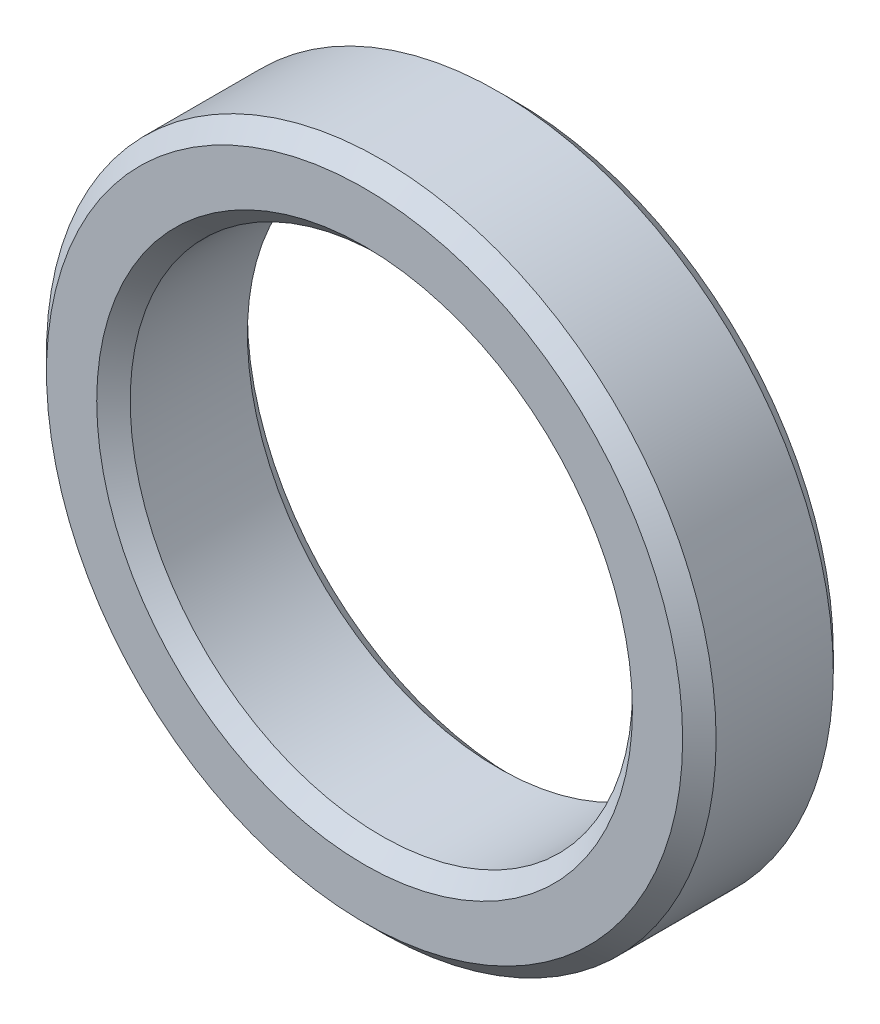
SolidWorks part; units mm, degrees
ref_plane "Front Plane" through (0, 0, 0) normal (0, 0, 1) x (1, 0, 0)
ref_plane "Top Plane" through (0, 0, 0) normal (0, 1, 0) x (1, 0, 0)
ref_plane "Right Plane" through (0, 0, 0) normal (1, 0, 0) x (0, 0, -1)
sketch "Sketch1" plane through (0, 0, 0) normal (0, 0, 1) x (1, 0, 0)
  circle A0 centre (0, 0) radius 10
  circle A1 centre (0, 0) radius 7.5
  dimension "D1" = 15
  dimension "D2" = 20
extrude "Boss-Extrude1" add sketch "Sketch1" along normal blind 4.5
chamfer "Chamfer1" distance 0.5 angle 45 4 edges at (7.5, 0, 0) (10, 0, 0) (7.5, 0, 4.5) (10, 0, 4.5)
